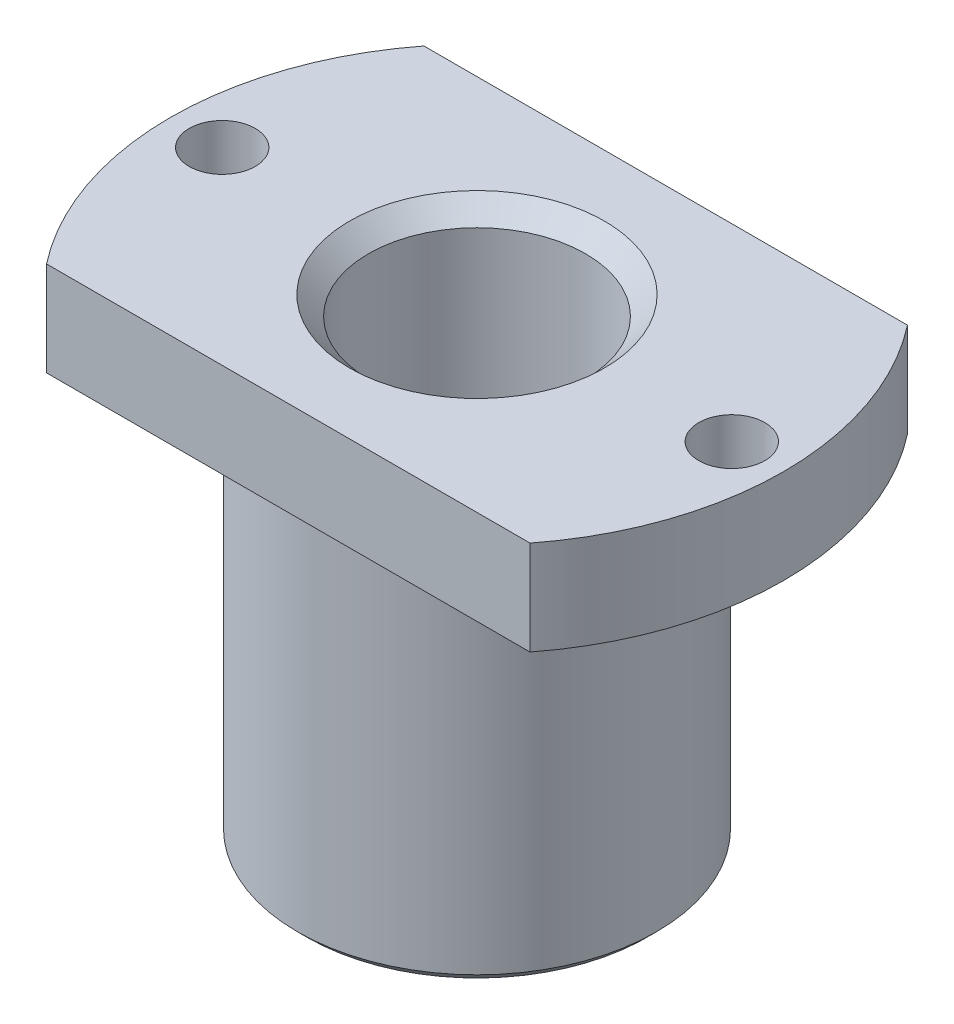
SolidWorks part; units mm, degrees
ref_plane "Front Plane" through (0, 0, 0) normal (0, 0, 1) x (1, 0, 0)
ref_plane "Top Plane" through (0, 0, 0) normal (0, 1, 0) x (1, 0, 0)
ref_plane "Right Plane" through (0, 0, 0) normal (1, 0, 0) x (0, 0, -1)
sketch "Sketch1" plane through (0, 0, 0) normal (0, 1, 0) x (1, 0, 0)
  circle A0 centre (0, 0) radius 19
  dimension "D1" = 38
extrude "Boss-Extrude1" add sketch "Sketch1" along normal blind 50
sketch "Sketch2" plane through (0, 50, 0) normal (0, 1, 0) x (1, 0, 0)
  circle A0 centre (0, 0) radius 32.5
  dimension "D1" = 65
extrude "Boss-Extrude2" add sketch "Sketch2" against normal blind 10
sketch "Sketch3" plane through (0, 0, 0) normal (0, -1, 0) x (1, 0, 0)
  circle A0 centre (0, 0) radius 11.5
  dimension "D1" = 23
extrude "Cut-Extrude1" cut sketch "Sketch3" against normal up to next
cosmetic thread "Cosmetic Thread2" parameters "D2"=69
sketch "Sketch4" plane through (0, 40, 0) normal (0, -1, 0) x (1, 0, 0)
  line L0 (0, 0) -> (-27, 0) construction
  circle A0 centre (0, 0) radius 27 construction
  circle A1 centre (-27, 0) radius 3.5
  dimension "D1" = 54
  dimension "D2" = 7
extrude "Cut-Extrude2" cut sketch "Sketch4" against normal through all
pattern_circular "CirPattern1" count 4 every 90 about axis through (0, 0, 0) along (0, 1, 0) of "Cut-Extrude1", "Cut-Extrude2"
chamfer "Chamfer1" distance 1 angle 45 1 edges at (0, 0, 19)
chamfer "Chamfer2" distance 2 angle 45 2 edges at (0, 0, -11.5) (0, 50, 11.5)
sketch "Sketch5" plane through (0, 50, 0) normal (0, 1, 0) x (1, 0, 0)
  line L0 (0, -20) -> (0, -33.1314) construction
  line L1 (-25.6174, -20) -> (25.6174, -20)
  line L2 (0, 0) -> (37.4746, 0) construction
  line L3 (0, 20) -> (0, 33.1314) construction
  line L4 (-25.6174, 20) -> (25.6174, 20)
  circle A0 centre (0, 0) radius 32.5 construction
  arc A1 (-25.6174, -20) -> (25.6174, -20) centre (0, 0) ccw
  arc A2 (-25.6174, 20) -> (25.6174, 20) centre (0, 0) cw
  dimension "D1" = 20
extrude "Cut-Extrude3" cut sketch "Sketch5" against normal up to next
